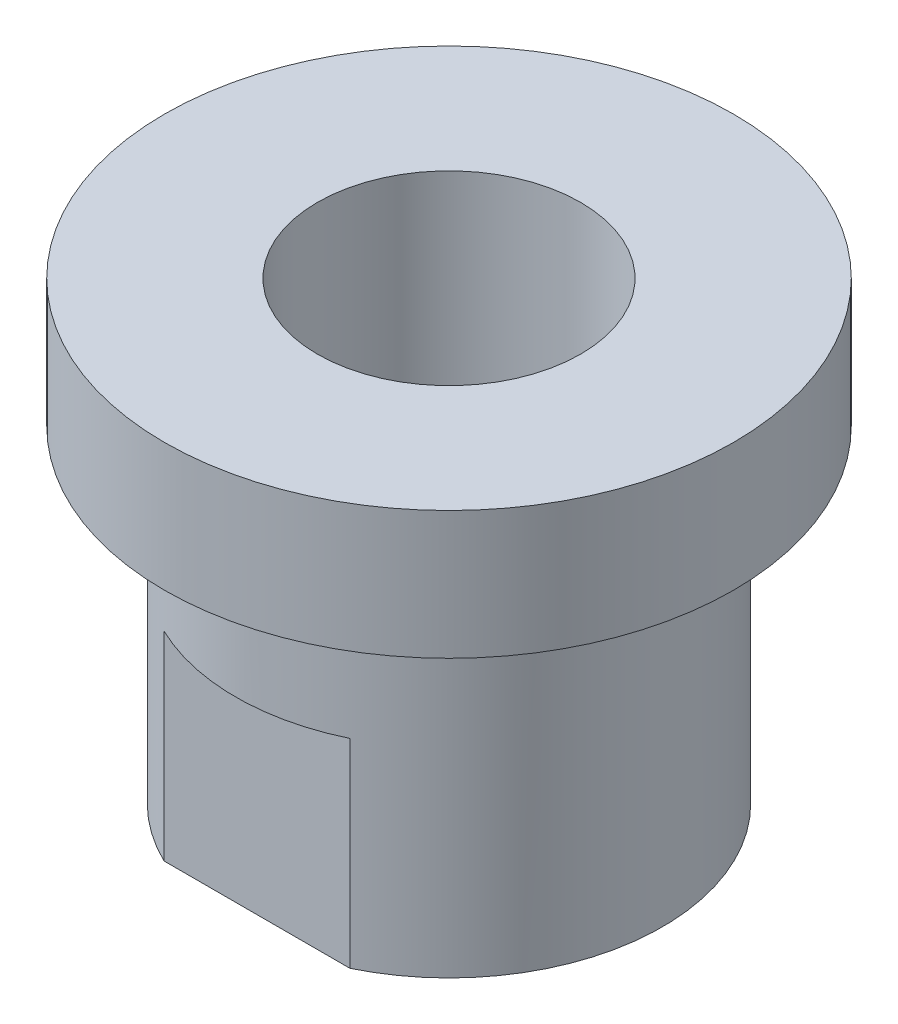
from build123d import *

# Parameters (mm, degrees)
SKETCH1_R               = 20
SKETCH1_R_2             = 9
BOSS_EXTRUDE1_DEPTH     = 32
SKETCH2_R               = 25
SKETCH2_R_2             = 15
CUT_EXTRUDE1_DEPTH      = 23
CUT_EXTRUDE2_DEPTH      = 43.708313008
CUT_EXTRUDE2_DEPTH_BACK = 43.708313008
SKETCH3_W               = 7.488703297
SKETCH3_H               = 21.290197802
M20X1_5_TAPPED_HOLE1_D  = 18.5


with BuildPart() as part:
    # Sketch1 → Boss-Extrude1 (new body)
    with BuildSketch(Plane(origin=(0, 0, 0), x_dir=(1, 0, 0), z_dir=(0, 1, 0))):
        with Locations(Location((0, 0, 0), (0, 0, 270))):
            Circle(SKETCH1_R)
        with Locations(Location((0, 0, 0), (0, 0, 270))):
            Circle(SKETCH1_R_2, mode=Mode.SUBTRACT)
    extrude(amount=BOSS_EXTRUDE1_DEPTH)

    # Sketch2 → Cut-Extrude1 (cut)
    with BuildSketch(Plane.XZ):
        Circle(SKETCH2_R)
        with Locations(Location((0, 0, 0), (0, 0, 270))):
            Circle(SKETCH2_R_2, mode=Mode.SUBTRACT)
    extrude(amount=-CUT_EXTRUDE1_DEPTH, mode=Mode.SUBTRACT)

    # Sketch3 → Cut-Extrude2 (cut, two sides: drawn at the far end of the back side and taken through both)
    with BuildSketch(Plane(origin=(0, 0, 0), x_dir=(0, 0, -1), z_dir=(1, 0, 0)).offset(-CUT_EXTRUDE2_DEPTH_BACK)):
        with Locations((-17.244351649, 3.354901099)):
            Rectangle(SKETCH3_W, SKETCH3_H)
        with Locations((17.244351649, 3.354901099)):
            Rectangle(SKETCH3_W, SKETCH3_H)
    extrude(amount=CUT_EXTRUDE2_DEPTH + CUT_EXTRUDE2_DEPTH_BACK, mode=Mode.SUBTRACT)

    # M20x1.5 Tapped Hole1 (through all)
    with Locations(Plane(origin=(0, 32, 0), x_dir=(1, 0, 0), z_dir=(0, 1, 0))):
        with Locations((0, 0)):
            Hole(M20X1_5_TAPPED_HOLE1_D / 2)


solid = part.part
